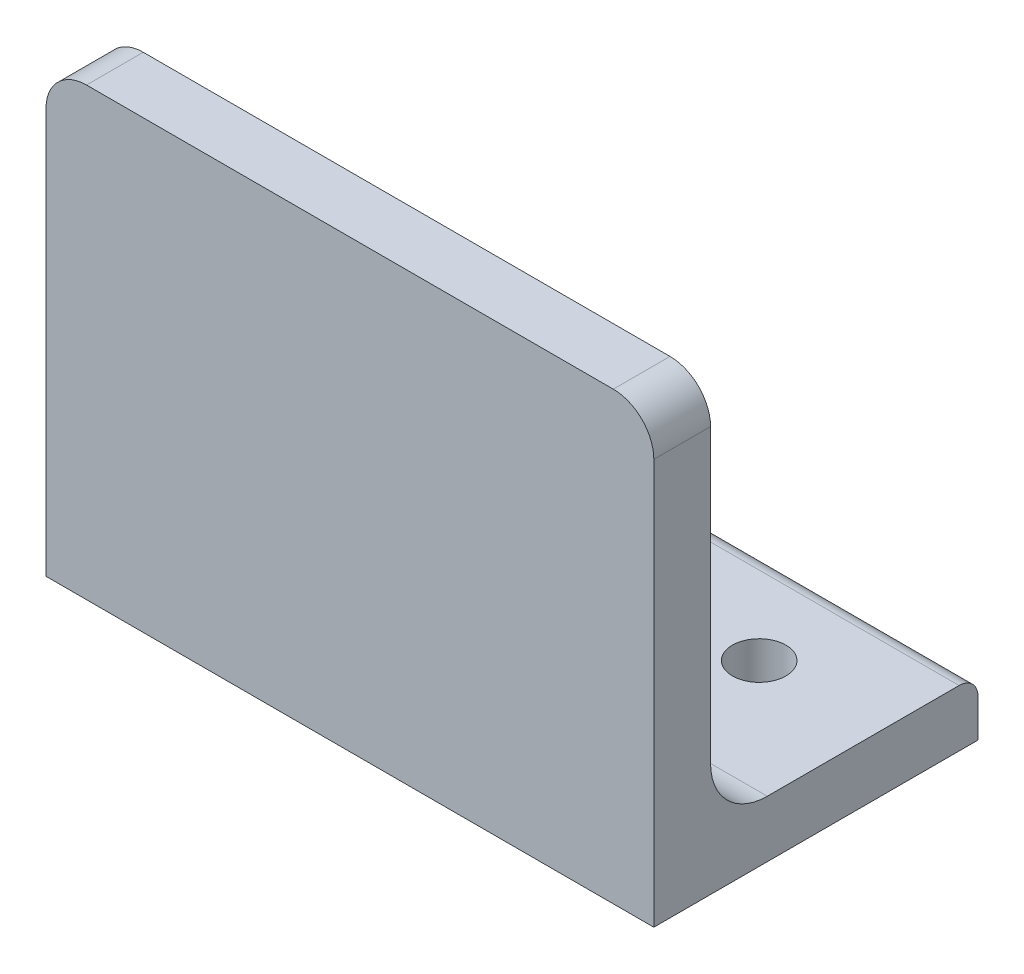
SolidWorks part; units mm, degrees
material "Q235"
ref_plane "Front Plane" through (0, 0, 0) normal (0, 0, 1) x (1, 0, 0)
ref_plane "Top Plane" through (0, 0, 0) normal (0, 1, 0) x (1, 0, 0)
ref_plane "Right Plane" through (0, 0, 0) normal (1, 0, 0) x (0, 0, -1)
sketch3d "3DSketch1"
  line L0 (0, 0, 0) -> (75, 0, 0)
  dimension "D1" = 75
other "Unequal angle 6.3-4(1)"
ref_plane "Plane1" through (0, 0, 0) normal (1, 0, 0) x (0, 1, 0)
sketch "Sketch11" plane through (0, 0, 0) normal (1, 0, 0) x (0, 1, 0)
  line L0 (63, 0) -> (0, 0)
  line L1 (0, 0) -> (0, -40)
  line L2 (60.6667, -7) -> (14, -7)
  line L3 (7, -14) -> (7, -37.6667)
  line L4 (63, 0) -> (63, -4.6667)
  line L5 (0, -40) -> (4.6667, -40)
  arc A0 (63, -4.6667) -> (60.6667, -7) centre (60.6667, -4.6667) cw
  arc A1 (4.6667, -40) -> (7, -37.6667) centre (4.6667, -37.6667) ccw
  arc A2 (14, -7) -> (7, -14) centre (14, -14) ccw
  point P2 (0, -20)
  point P13 (31.5, 0)
  point P14 (0, 0)
  dimension "r1" = 2.3333
  dimension "r" = 7
  dimension "a" = 63
  dimension "d" = 7
  dimension "b" = 40
hole_wizard "M6 Clearance Hole1" positions "Sketch5" profile "Sketch6" hole size "M6" standard "GB"
sketch "Sketch5" plane through (0, 0, 0) normal (0, 1, 0) x (1, 0, 0)
  line L0 (75, 0) -> (0, 0) construction
  line L3 (0, 37.6667) -> (0, 14) construction
  line L4 (75, 37.6667) -> (75, 14) construction
  point P0 (15, 28)
  point P2 (60, 28)
  dimension "D1" = 28
  dimension "D2" = 15
  dimension "D3" = 15
sketch "Sketch6" plane through (15, 0, -28) normal (1, 0, 0) x (0, 0, -1)
  line L0 (0, 0) -> (0, 21.9828)
  line L1 (0, 21.9828) -> (3.3, 20)
  line L2 (3.3, 20) -> (3.3, 0)
  line L5 (3.3, 0) -> (0, 0)
  line L10 (0, 21.9828) -> (-3.3, 20) construction
  line L11 (0, -6.35) -> (0, 107.95) construction
  dimension "孔直径" = 6.6
  dimension "孔深度" = 20
  dimension "导头角度" = 118
sketch "Sketch8" plane through (75, 0, 0) normal (1, 0, 0) x (0, 0, -1)
  line L0 (7, 14) -> (7, 60.6667) construction
  line L1 (-7, 71) -> (7, 71)
  line L2 (-7, 71) -> (-7, 55)
  line L3 (-7, 55) -> (7, 55)
  line L4 (7, 71) -> (7, 55)
  line L5 (-7, 71) -> (7, 55) construction
  line L6 (-7, 55) -> (7, 71) construction
  line L7 (0, 0) -> (40, 0) construction
  point P0 (0, 63)
  dimension "D1" = 55
extrude "Cut-Extrude1" cut sketch "Sketch8" against normal through all both and the other way through all
fillet "Fillet1" radius 5 2 edges at (0, 55, -3.5) (75, 55, -3.5)
